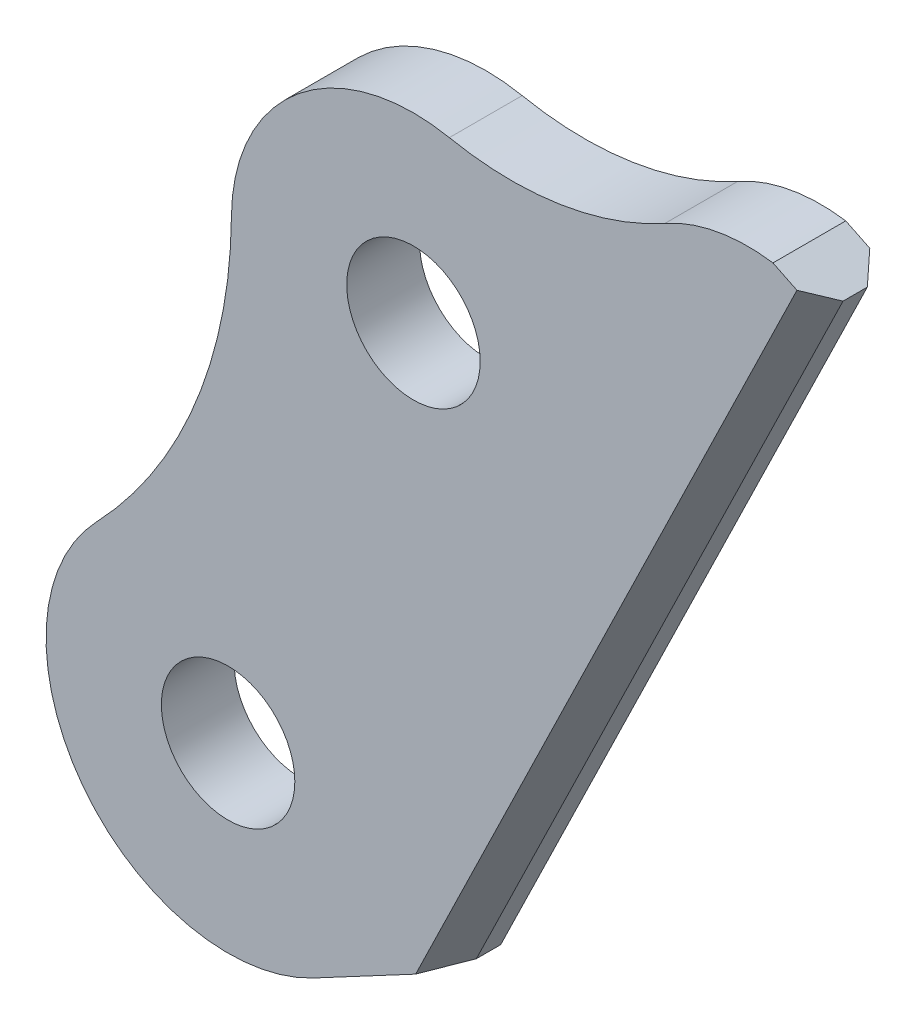
from build123d import *

# Parameters (mm, degrees)
SKETCH1_R           = 27.5
BOSS_EXTRUDE1_DEPTH = 30
CHAMFER1_SIZE       = 10


with BuildPart() as part:
    # Sketch1 → Boss-Extrude1 (new body)
    with BuildSketch(Plane.XY):
        with BuildLine():
            Line((92.3, -35.8), (243.373525417, 274.385312067))
            Line((243.373525417, 274.385312067), (224.493722277, 283.580584405))
            ThreePointArc((224.493722277, 283.580584405), (201.609043027, 283.221639878), (180.06339689, 275.500077984))
            ThreePointArc((180.06339689, 275.500077984), (136.851269704, 260.619417011), (91.159540852, 261.61335942))
            ThreePointArc((91.159540852, 261.61335942), (29.078225578, 246.293169038), (1.375741332, 188.661838097))
            ThreePointArc((1.375741332, 188.661838097), (-13.312623389, 114.954388214), (-54.16864079, 51.87252023))
            ThreePointArc((-54.16864079, 51.87252023), (-59.782430884, -45.288640491), (35.270014595, -66.189319912))
            Line((35.270014595, -66.189319912), (92.3, -35.8))
        make_face()
        with Locations((76.373525417, 188.085312067)):
            Circle(SKETCH1_R, mode=Mode.SUBTRACT)
        Circle(SKETCH1_R, mode=Mode.SUBTRACT)
    extrude(amount=BOSS_EXTRUDE1_DEPTH)

    # Chamfer1
    chamfer1_edges = [part.edges().sort_by_distance(p)[0] for p in [
        (167.836762709, 119.292656033, 0),
        (167.836762709, 119.292656033, 30),
    ]]
    chamfer(chamfer1_edges, length=CHAMFER1_SIZE)


solid = part.part
